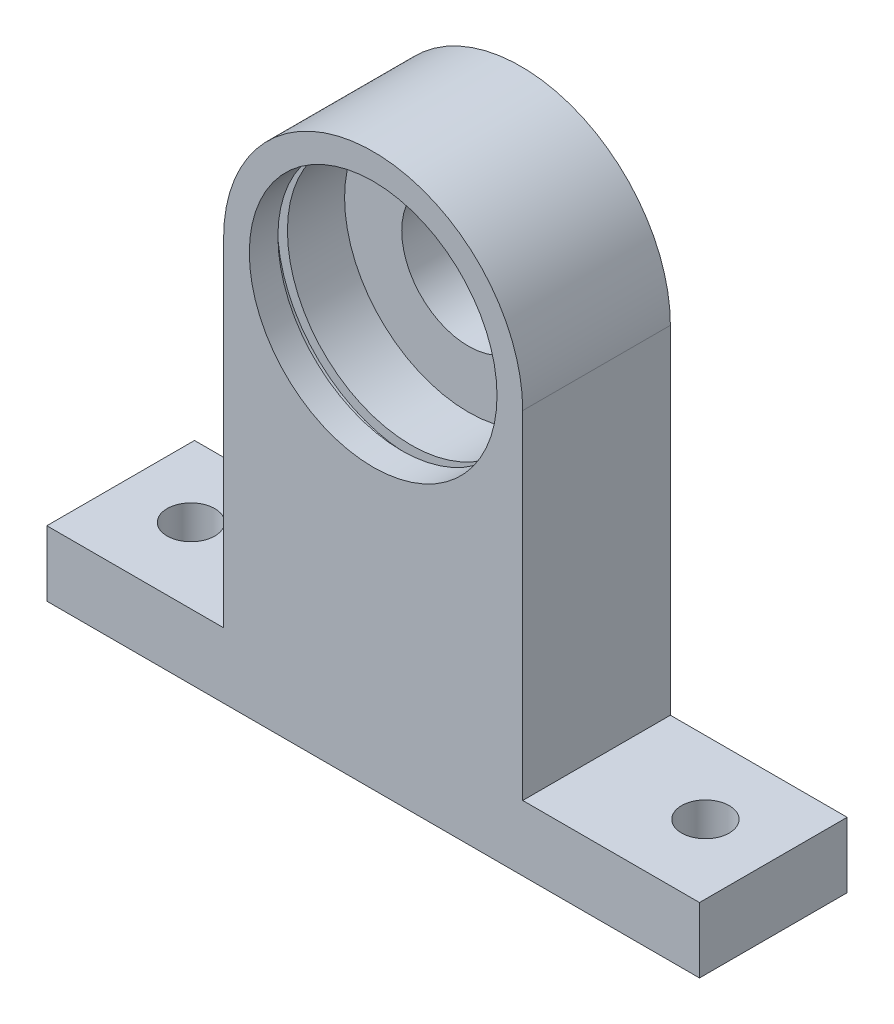
SolidWorks part; units mm, degrees
ref_plane "Front Plane" through (0, 0, 0) normal (0, 0, 1) x (1, 0, 0)
ref_plane "Top Plane" through (0, 0, 0) normal (0, 1, 0) x (1, 0, 0)
ref_plane "Right Plane" through (0, 0, 0) normal (1, 0, 0) x (0, 0, -1)
sketch "Sketch1" plane through (0, 0, 0) normal (0, 0, 1) x (1, 0, 0)
  line L0 (-31.3969, 0.4439) -> (-31.3969, -70.8886)
  line L1 (-31.3969, -70.8886) -> (-68.5067, -70.8886)
  line L2 (-68.5067, -70.8886) -> (-68.5067, -84.6086)
  line L3 (-68.5067, -84.6086) -> (68.5067, -84.6086)
  line L5 (68.5067, -70.8886) -> (68.5067, -84.6086)
  line L6 (31.3969, -70.8886) -> (68.5067, -70.8886)
  line L7 (31.3969, 0.4439) -> (31.3969, -70.8886)
  circle A0 centre (0, 0) radius 12.5
  circle A1 centre (0, 0) radius 31.3969
extrude "Boss-Extrude1" add sketch "Sketch1" along normal blind 31 contours A1 A0 | A1 L0 L1 L2 L3 L5 L6 L7
sketch "Sketch2" plane through (0, -70.8886, 0) normal (0, 1, 0) x (1, 0, 0)
  line L0 (0, 0) -> (0, -31)
  line L1 (-31.3969, -31) -> (31.3969, -31) construction
  circle A0 centre (54, -15.251) radius 5
  circle A1 centre (-54, -15.251) radius 5
  dimension "D1" = 54
  dimension "D2" = 10
extrude "Cut-Extrude1" cut sketch "Sketch2" against normal blind 31 contours A0 | A1
sketch "Sketch3" plane through (0, 0, 0) normal (0, 0, -1) x (-1, 0, 0)
  circle A0 centre (0, 0) radius 14
  dimension "D1" = 28
extrude "Cut-Extrude2" cut sketch "Sketch3" against normal through all
sketch "Sketch5" plane through (0, 0, 31) normal (0, 0, 1) x (1, 0, 0)
  circle A0 centre (0, 0) radius 26
  dimension "D1" = 52
extrude "Cut-Extrude4" cut sketch "Sketch5" against normal blind 20
ref_plane "Plane1" through (0, 0, 23) normal (0, 0, 1) x (1, 0, 0)
sketch "Sketch6" plane through (0, 0, 23) normal (0, 0, 1) x (1, 0, 0)
  circle A0 centre (0, 0) radius 28.1
  dimension "D1" = 56.2
extrude "Cut-Extrude5" cut sketch "Sketch6" along normal blind 2
